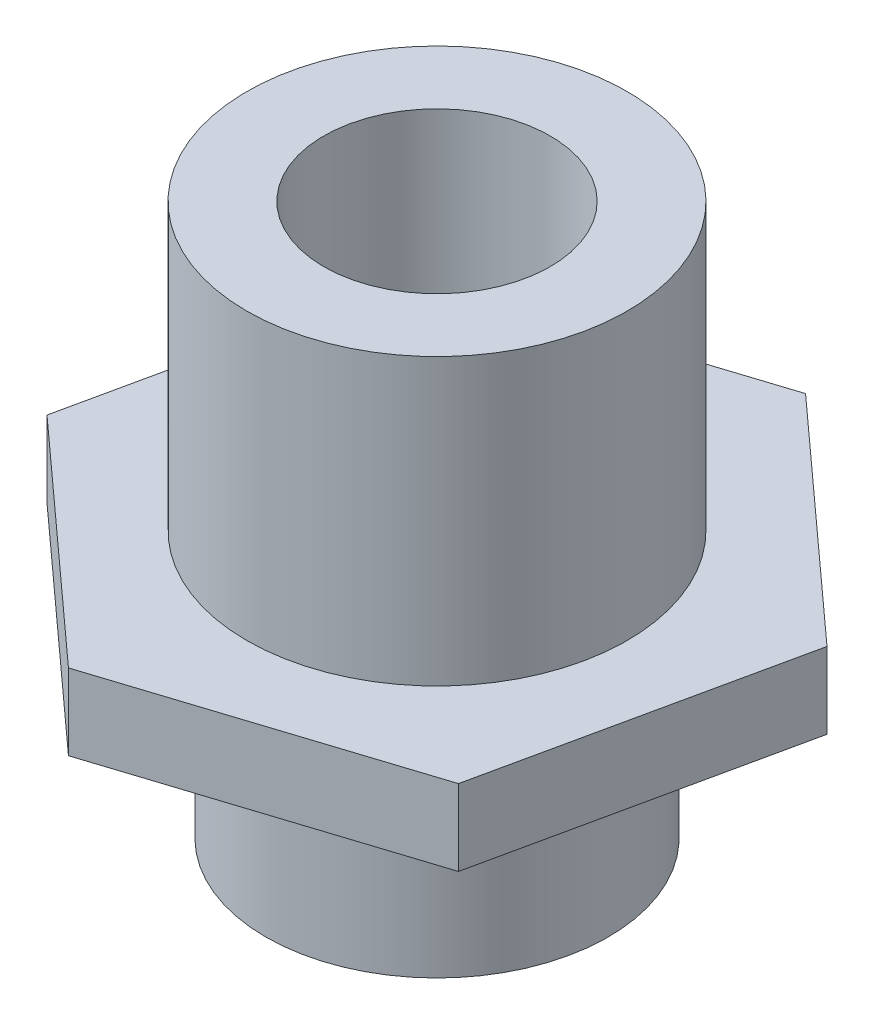
from build123d import *

# Parameters (mm, degrees)
SKETCH1_R           = 9
SKETCH1_R_2         = 6
BOSS_EXTRUDE1_DEPTH = 10
SKETCH2_R           = 5.955432099
BOSS_EXTRUDE2_DEPTH = 4
SKETCH3_R           = 10
SKETCH3_R_2         = 5.955432099
BOSS_EXTRUDE3_DEPTH = 15


with BuildPart() as part:
    # Sketch1 → Boss-Extrude1 (new body)
    with BuildSketch(Plane(origin=(0, 0, 0), x_dir=(1, 0, 0), z_dir=(0, 1, 0))):
        with Locations(Location((0, 0, 0), (0, 0, 270))):
            Circle(SKETCH1_R)
        with Locations(Location((0, 0, 0), (0, 0, 270))):
            Circle(SKETCH1_R_2, mode=Mode.SUBTRACT)
    extrude(amount=BOSS_EXTRUDE1_DEPTH)


with BuildPart() as body_2:
    # Sketch2 → Boss-Extrude2 (new body)
    with BuildSketch(Plane(origin=(0, 10, 0), x_dir=(1, 0, 0), z_dir=(0, 1, 0))):
        Polygon((-12.076383081, 10.948356194), (-15.519746134, -4.984276437), (-3.443363053, -15.93263263), (12.076383081, -10.948356194), (15.519746134, 4.984276437), (3.443363053, 15.93263263), align=None)
        with Locations(Location((0, 0, 0), (0, 0, 270))):
            Circle(SKETCH2_R, mode=Mode.SUBTRACT)
    extrude(amount=BOSS_EXTRUDE2_DEPTH)

    # Sketch3 → Boss-Extrude3 (add)
    with BuildSketch(Plane(origin=(0, 14, 0), x_dir=(1, 0, 0), z_dir=(0, 1, 0))):
        with Locations(Location((0, 0, 0), (0, 0, 270))):
            Circle(SKETCH3_R)
        with Locations(Location((0, 0, 0), (0, 0, 270))):
            Circle(SKETCH3_R_2, mode=Mode.SUBTRACT)
    extrude(amount=BOSS_EXTRUDE3_DEPTH)


solid = Compound([part.part, body_2.part])
